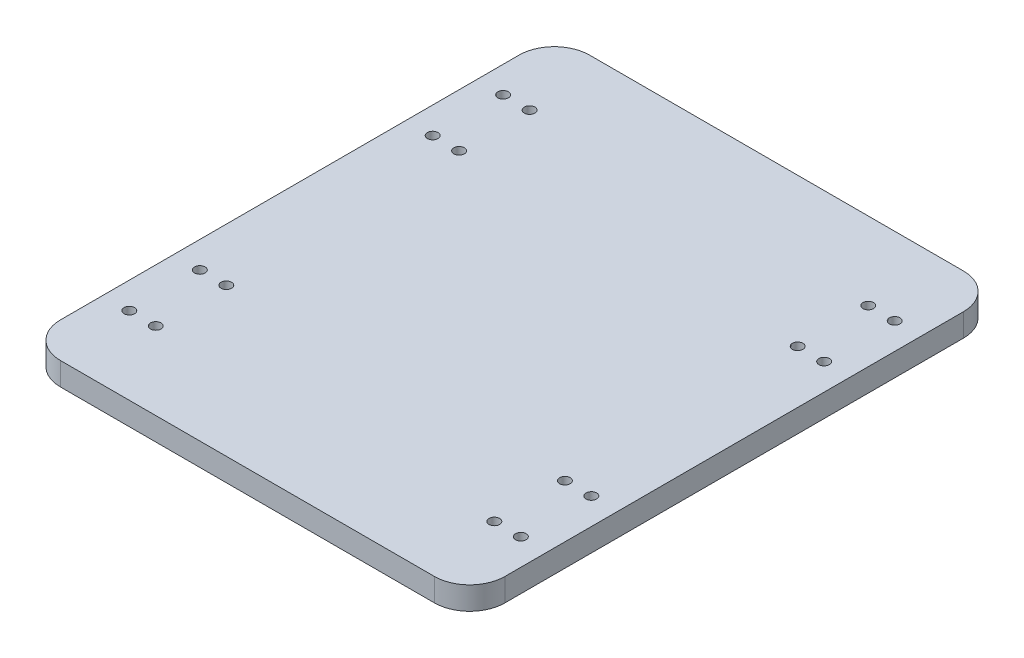
from build123d import *

# Parameters (mm, degrees)
SKETCH1_W               = 126
SKETCH1_H               = 150
BOSS_EXTRUDE1_DEPTH     = 6.5
SKETCH2_R               = 1.5
CUT_EXTRUDE1_DEPTH      = 10
MIRROR2_COPY_1_SKETCH_R = 1.5
MIRROR2_COPY_1_DEPTH    = 10
FILLET1_R               = 10


with BuildPart() as part:
    # Sketch1 → Boss-Extrude1 (new body)
    with BuildSketch(Plane(origin=(0, 0, 0), x_dir=(1, 0, 0), z_dir=(0, 1, 0))):
        Rectangle(SKETCH1_W, SKETCH1_H)
    extrude(amount=BOSS_EXTRUDE1_DEPTH)

    # Sketch2 → Cut-Extrude1 (cut)
    with BuildSketch(Plane(origin=(0, 6.5, 0), x_dir=(1, 0, 0), z_dir=(0, 1, 0))):
        with Locations(Location((-55.5, 33, 0), (0, 0, 270))):
            Circle(SKETCH2_R)
        with Locations(Location((-48, 33, 0), (0, 0, 90))):
            Circle(SKETCH2_R)
        with Locations(Location((-48, 53, 0), (0, 0, 270))):
            Circle(SKETCH2_R)
        with Locations(Location((-55.5, 53, 0), (0, 0, 90))):
            Circle(SKETCH2_R)
    cut_extrude1 = extrude(amount=-CUT_EXTRUDE1_DEPTH, mode=Mode.SUBTRACT)

    # Mirror1: Cut-Extrude1 across plane
    add(cut_extrude1.mirror(Plane(origin=(0, 0, 0), x_dir=(0, 0, 1), z_dir=(1, 0, 0))), mode=Mode.SUBTRACT)

    # Mirror2: Cut-Extrude1 across plane
    add(cut_extrude1.mirror(Plane.XY), mode=Mode.SUBTRACT)

    # Mirror2 copy 1 sketch → Mirror2 copy 1 (cut)
    with BuildSketch(Plane(origin=(0, 6.5, 0), x_dir=(-1, 0, 0), z_dir=(0, 1, 0))):
        with Locations(Location((-55.5, 33, 0), (0, 0, 270))):
            Circle(MIRROR2_COPY_1_SKETCH_R)
        with Locations(Location((-48, 33, 0), (0, 0, 90))):
            Circle(MIRROR2_COPY_1_SKETCH_R)
        with Locations(Location((-48, 53, 0), (0, 0, 270))):
            Circle(MIRROR2_COPY_1_SKETCH_R)
        with Locations(Location((-55.5, 53, 0), (0, 0, 90))):
            Circle(MIRROR2_COPY_1_SKETCH_R)
    extrude(amount=-MIRROR2_COPY_1_DEPTH, mode=Mode.SUBTRACT)

    # Fillet1
    fillet1_edges = [part.edges().sort_by_distance(p)[0] for p in [
        (63, 3.25, 75),
        (-63, 3.25, 75),
        (-63, 3.25, -75),
        (63, 3.25, -75),
    ]]
    fillet(fillet1_edges, radius=FILLET1_R)


solid = part.part
